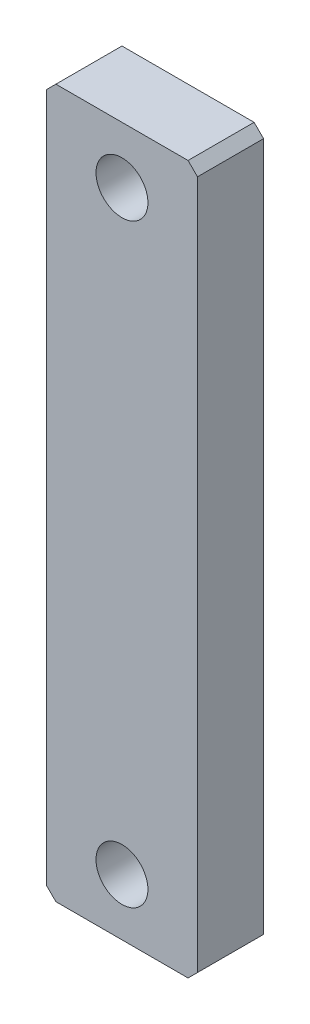
from build123d import *

# Parameters (mm, degrees)
SKETCH1_W            = 16
SKETCH1_H            = 75
BOSS_EXTRUDE1_DEPTH  = 7
CHAMFER5_SIZE        = 1
M5_CLEARANCE_HOLE1_D = 5.5


with BuildPart() as part:
    # Sketch1 → Boss-Extrude1 (new body)
    with BuildSketch(Plane.XY):
        Rectangle(SKETCH1_W, SKETCH1_H)
    extrude(amount=BOSS_EXTRUDE1_DEPTH)

    # Chamfer5
    chamfer5_edges = [part.edges().sort_by_distance(p)[0] for p in [
        (8, -37.5, 3.5),
        (-8, -37.5, 3.5),
        (-8, 37.5, 3.5),
        (8, 37.5, 3.5),
    ]]
    chamfer(chamfer5_edges, length=CHAMFER5_SIZE)

    # M5 Clearance Hole1 (through all)
    with Locations(Plane.XY.offset(7)):
        with Locations((0, 31.5), (0, -31.5)):
            Hole(M5_CLEARANCE_HOLE1_D / 2)


solid = part.part
